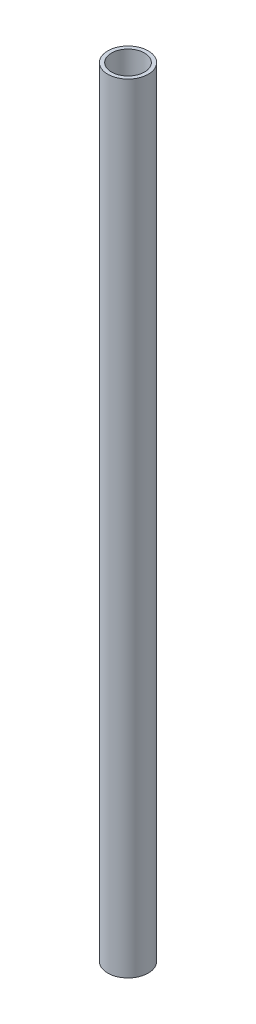
SolidWorks part; units mm, degrees
material "Q235B"
ref_plane "Front Plane" through (0, 0, 0) normal (0, 0, 1) x (1, 0, 0)
ref_plane "Top Plane" through (0, 0, 0) normal (0, 1, 0) x (1, 0, 0)
ref_plane "Right Plane" through (0, 0, 0) normal (1, 0, 0) x (0, 0, -1)
sketch "草图1" plane through (0, 0, 0) normal (0, 0, 1) x (1, 0, 0)
  line L0 (0, 0) -> (0, 1460)
  dimension "D1" = 1460
other "Gb/t 6728-2002 round tube 76×7(1)"
ref_plane "Plane1" through (0, 0, 0) normal (0, 1, 0) x (-1, 0, 0)
sketch "Sketch1" plane through (0, 0, 0) normal (0, 1, 0) x (-1, 0, 0)
  circle A0 centre (0, 0) radius 31
  circle A1 centre (0, 0) radius 38
  point P3 (0, 0)
  dimension "In_dia" = 62
  dimension "Out_dia" = 76
